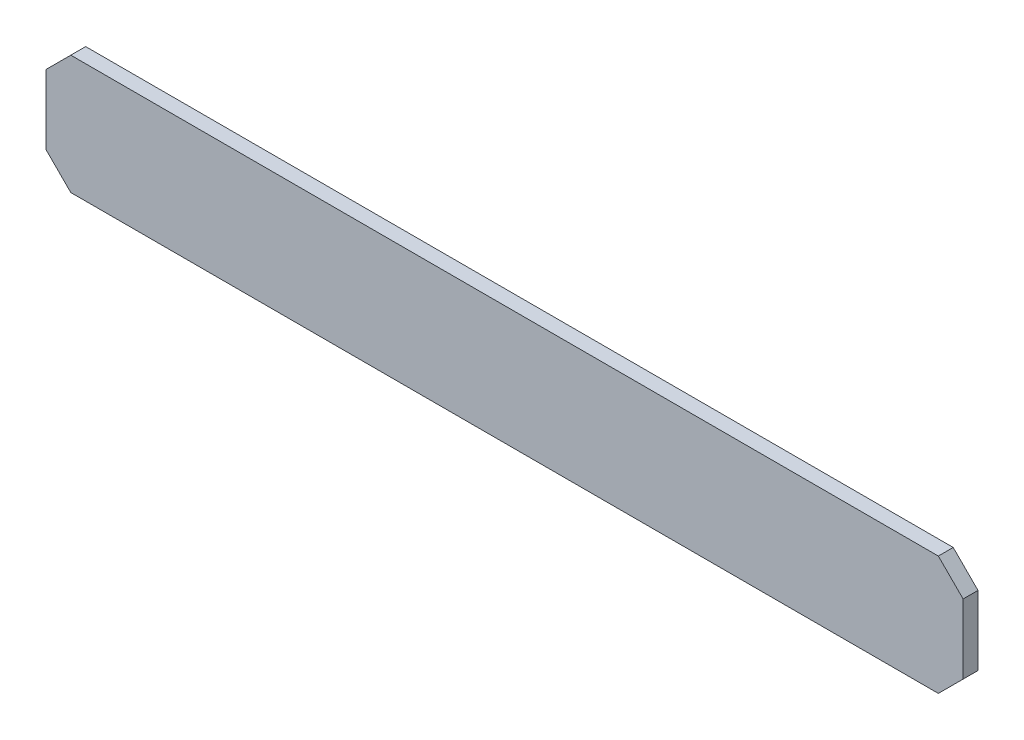
SolidWorks part; units mm, degrees
material "Q235A"
ref_plane "前视基准面" through (0, 0, 0) normal (0, 0, 1) x (1, 0, 0)
ref_plane "上视基准面" through (0, 0, 0) normal (0, 1, 0) x (1, 0, 0)
ref_plane "右视基准面" through (0, 0, 0) normal (1, 0, 0) x (0, 0, -1)
sketch "草图1" plane through (0, 0, 0) normal (0, 0, 1) x (1, 0, 0)
  line L0 (-92.5, 19) -> (-87.5, 24)
  line L1 (-87.5, 24) -> (87.5, 24)
  line L2 (-92.5, 19) -> (-92.5, 5)
  line L3 (-87.5, 0) -> (87.5, 0)
  line L4 (92.5, 19) -> (92.5, 5)
  line L5 (-92.5, 5) -> (-87.5, 0)
  line L6 (87.5, 0) -> (92.5, 5)
  line L7 (87.5, 24) -> (92.5, 19)
  point P0 (-92.5, 24)
  point P1 (92.5, 0)
  point P2 (-92.5, 0)
  point P3 (92.5, 24)
  point P12 (-92.5, 12)
  dimension "D1" = 5
  dimension "D2" = 5
  dimension "D3" = 5
  dimension "D4" = 5
  dimension "D5" = 5
  dimension "D6" = 5
  dimension "D7" = 5
  dimension "D8" = 5
  dimension "D9" = 185
  dimension "D10" = 24
extrude "凸台-拉伸1" add sketch "草图1" along normal blind 3
